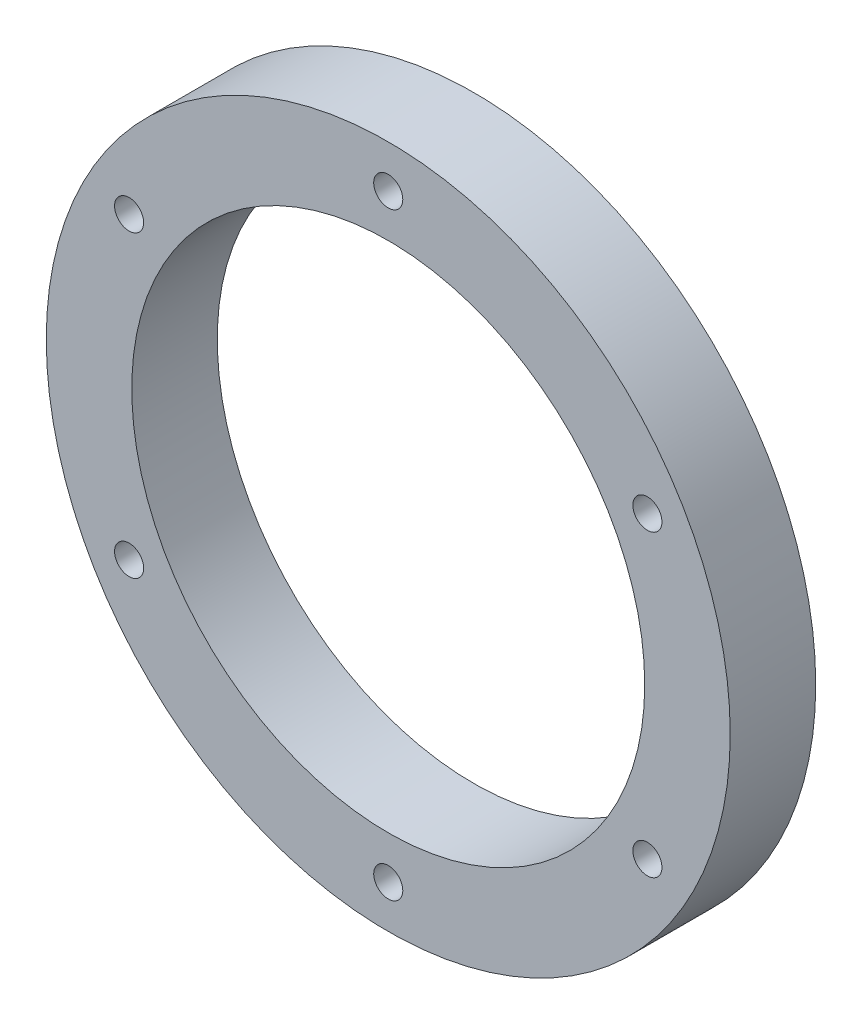
SolidWorks part; units mm, degrees
ref_plane "Front Plane" through (0, 0, 0) normal (0, 0, 1) x (1, 0, 0)
ref_plane "Top Plane" through (0, 0, 0) normal (0, 1, 0) x (1, 0, 0)
ref_plane "Right Plane" through (0, 0, 0) normal (1, 0, 0) x (0, 0, -1)
sketch "Sketch1" plane through (0, 0, 0) normal (0, 0, 1) x (1, 0, 0)
  circle A0 centre (0, 0) radius 80
  circle A1 centre (0, 0) radius 60
extrude "Boss-Extrude1" add sketch "Sketch1" along normal blind 20
sketch "Sketch2" plane through (0, 0, 20) normal (0, 0, 1) x (1, 0, 0)
  circle A1 centre (0, 70) radius 3.95
  circle A2 centre (60.6218, 35) radius 3.95
  circle A3 centre (60.6218, -35) radius 3.95
  circle A4 centre (0, -70) radius 3.95
  circle A5 centre (-60.6218, -35) radius 3.95
  circle A6 centre (-60.6218, 35) radius 3.95
  point P18 (0, 0)
  dimension "D1" = 6
hole_wizard "M8 Tapped Hole1" positions "3DSketch2" profile "Sketch4" tap size "M8" standard "Gb"
sketch3d "3DSketch2"
  point P0 (0, 70, 20)
  point P3 (60.6218, 35, 20)
  point P6 (60.6218, -35, 20)
  point P9 (0, -70, 20)
  point P12 (-60.6218, -35, 20)
  point P15 (-60.6218, 35, 20)
sketch "Sketch4" plane through (0, 70, 20) normal (1, 0, 0) x (0, -1, 0)
  line L0 (0, 0) -> (0, 20.0429)
  line L1 (0, 20.0429) -> (3.4, 18)
  line L2 (3.4, 18) -> (3.4, 0)
  line L5 (3.4, 0) -> (0, 0)
  line L10 (0, 20.0429) -> (-3.4, 18) construction
  line L11 (0, -6.35) -> (0, 107.95) construction
  dimension "螺纹孔钻头直径" = 6.8
  dimension "螺纹孔钻头深度" = 18
  dimension "导头角度" = 118
cosmetic thread "Hole Cosmetic Thread1" parameters "D1"=10, "D2"=8
cosmetic thread "Hole Cosmetic Thread2" parameters "D1"=10, "D2"=8
cosmetic thread "Hole Cosmetic Thread3" parameters "D1"=10, "D2"=8
cosmetic thread "Hole Cosmetic Thread4" parameters "D1"=10, "D2"=8
cosmetic thread "Hole Cosmetic Thread5" parameters "D1"=10, "D2"=8
cosmetic thread "Hole Cosmetic Thread6" parameters "D1"=10, "D2"=8
